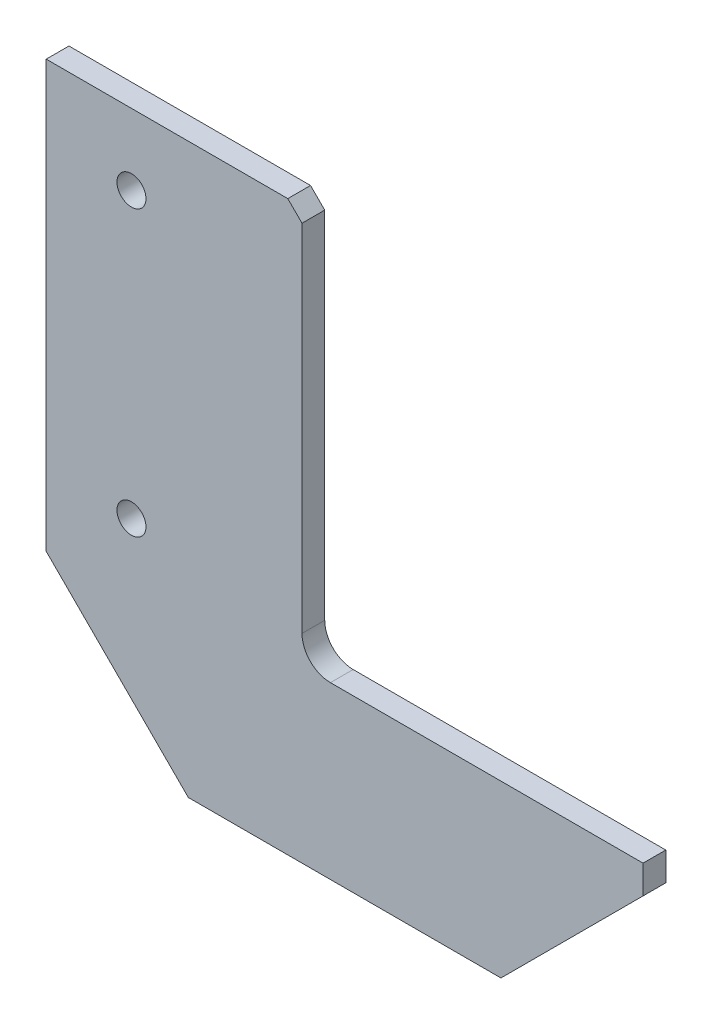
SolidWorks part; units mm, degrees
material "1023 碳钢板 (SS)"
ref_plane "Front Plane" through (0, 0, 0) normal (0, 0, 1) x (1, 0, 0)
ref_plane "Top Plane" through (0, 0, 0) normal (0, 1, 0) x (1, 0, 0)
ref_plane "Right Plane" through (0, 0, 0) normal (1, 0, 0) x (0, 0, -1)
sketch "Sketch1" plane through (0, 0, 0) normal (0, 0, 1) x (1, 0, 0)
  line L1 (105, 100) -> (-105, 100)
  line L2 (105, 100) -> (105, -100)
  line L3 (105, -100) -> (-105, -100)
  line L4 (-105, 100) -> (-105, -100)
  line L5 (105, 100) -> (-105, -100) construction
  line L6 (105, -100) -> (-105, 100) construction
  point P0 (0, 0)
  dimension "D1" = 210
  dimension "D2" = 200
extrude "Boss-Extrude1" add sketch "Sketch1" along normal blind 8
chamfer "Chamfer1" distance 50 angle 45 2 edges at (105, -100, 4) (-105, -100, 4)
sketch "Sketch2" plane through (0, 0, 8) normal (0, 0, 1) x (1, 0, 0)
  line L0 (105, 100) -> (-105, 100) construction
  line L1 (-105, 100) -> (-105, -50) construction
  circle A0 centre (-75, 75.01) radius 5
  circle A1 centre (-75, -24.99) radius 5
  dimension "D4" = 10
  dimension "D1" = 100
  dimension "D2" = 24.99
  dimension "D3" = 30
hole_wizard "M12 Tapped Hole1" positions "Sketch3" profile "Sketch4" tap size "M12" standard "ISO"
sketch "Sketch3" plane through (0, 0, 8) normal (0, 0, 1) x (1, 0, 0)
  point P0 (-75, 75.01)
  point P3 (-75, -24.99)
sketch "Sketch4" plane through (-75, 75.01, 8) normal (1, 0, 0) x (0, -1, 0)
  line L0 (0, 0) -> (0, 32.3144)
  line L1 (0, 32.3144) -> (5.1, 29.25)
  line L2 (5.1, 29.25) -> (5.1, 0)
  line L5 (5.1, 0) -> (0, 0)
  line L10 (0, 32.3144) -> (-5.1, 29.25) construction
  line L11 (0, -6.35) -> (0, 107.95) construction
  dimension "螺纹孔钻头直径" = 10.2
  dimension "螺纹孔钻头深度" = 29.25
  dimension "导头角度" = 118
cosmetic thread "Hole thread line 1" parameters "D1"=24, "D2"=12
cosmetic thread "Hole thread line 2" parameters "D1"=24, "D2"=12
sketch "Sketch5" plane through (0, 0, 8) normal (0, 0, 1) x (1, 0, 0)
  line L0 (105, 100) -> (-105, 100) construction
  line L1 (-15, -40) -> (165.5483, -40)
  line L2 (-15, -40) -> (-15, 125.8297)
  line L3 (-15, 125.8297) -> (165.5483, 125.8297)
  line L4 (165.5483, -40) -> (165.5483, 125.8297)
  line L5 (-15, -40) -> (165.5483, 125.8297) construction
  line L6 (-15, 125.8297) -> (165.5483, -40) construction
  line L7 (105, -50) -> (105, 100) construction
  point P0 (75.2741, 42.9148)
  dimension "D1" = 140
  dimension "D2" = 120
extrude "Cut-Extrude1" cut sketch "Sketch5" against normal blind 8
chamfer "Chamfer2" distance 5 angle 45 1 edges at (-15, 100, 4)
fillet "Fillet1" radius 10 1 edges at (-15, -40, 4)
